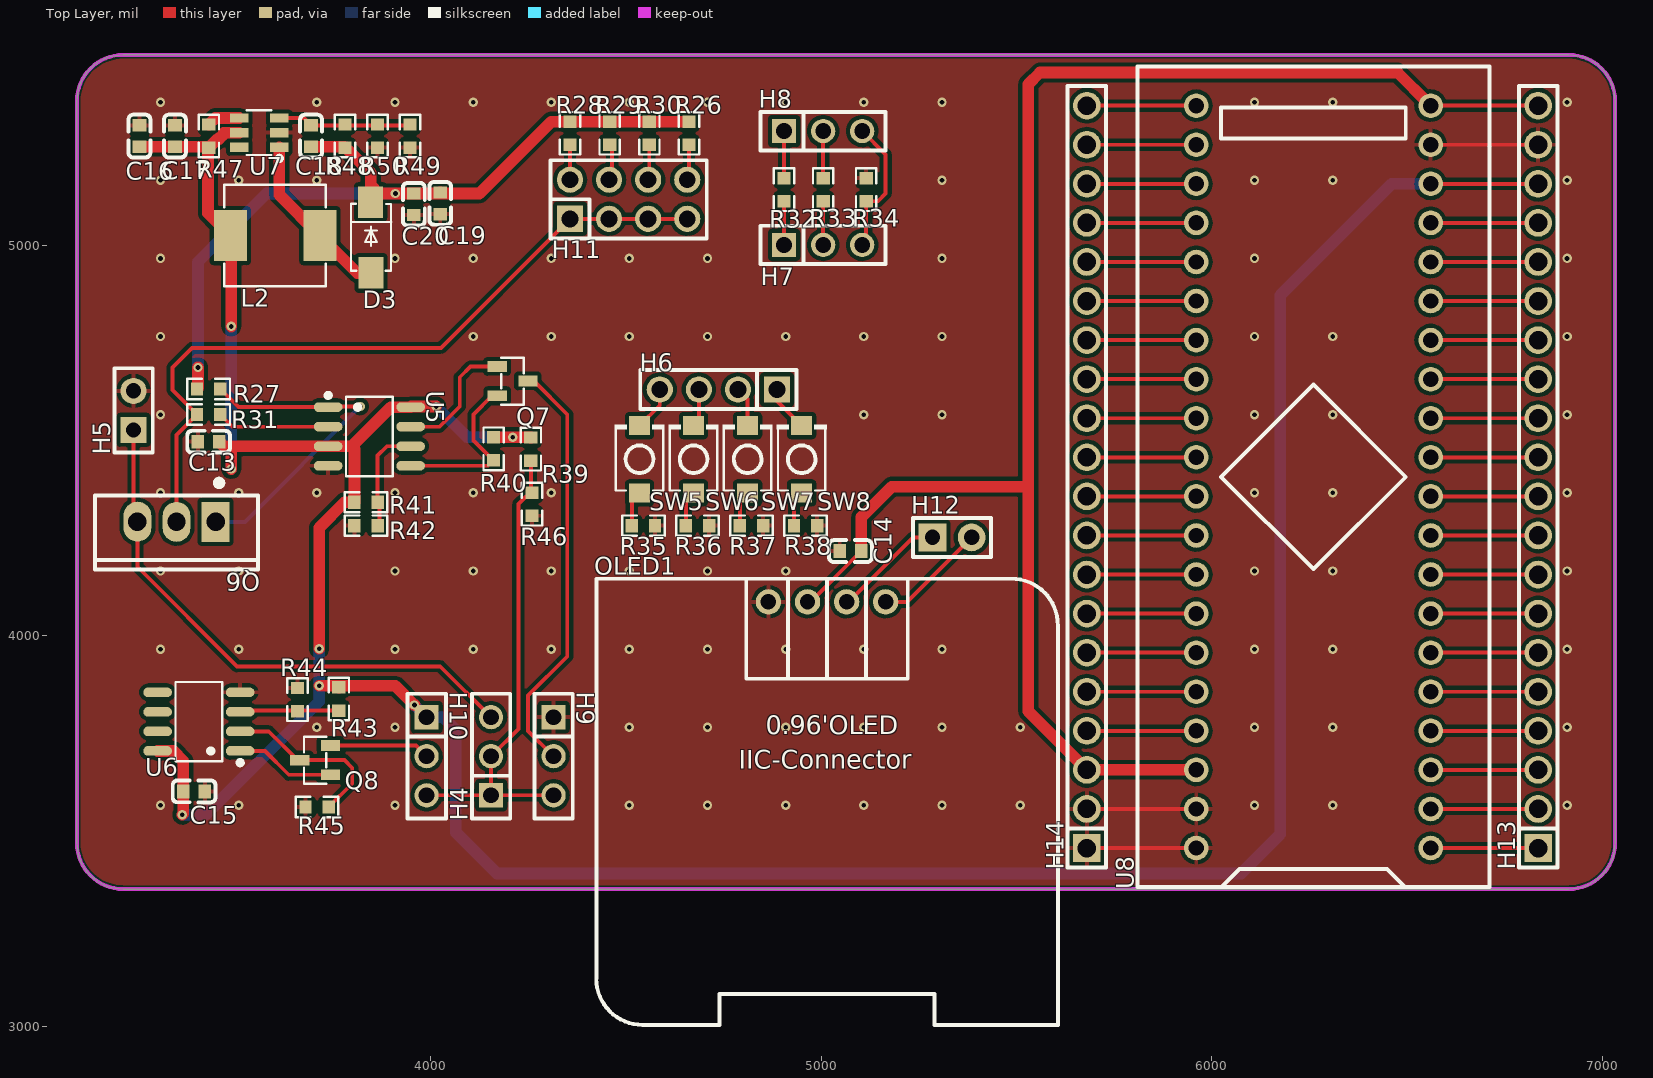
[diagram p0: Top Layer view]
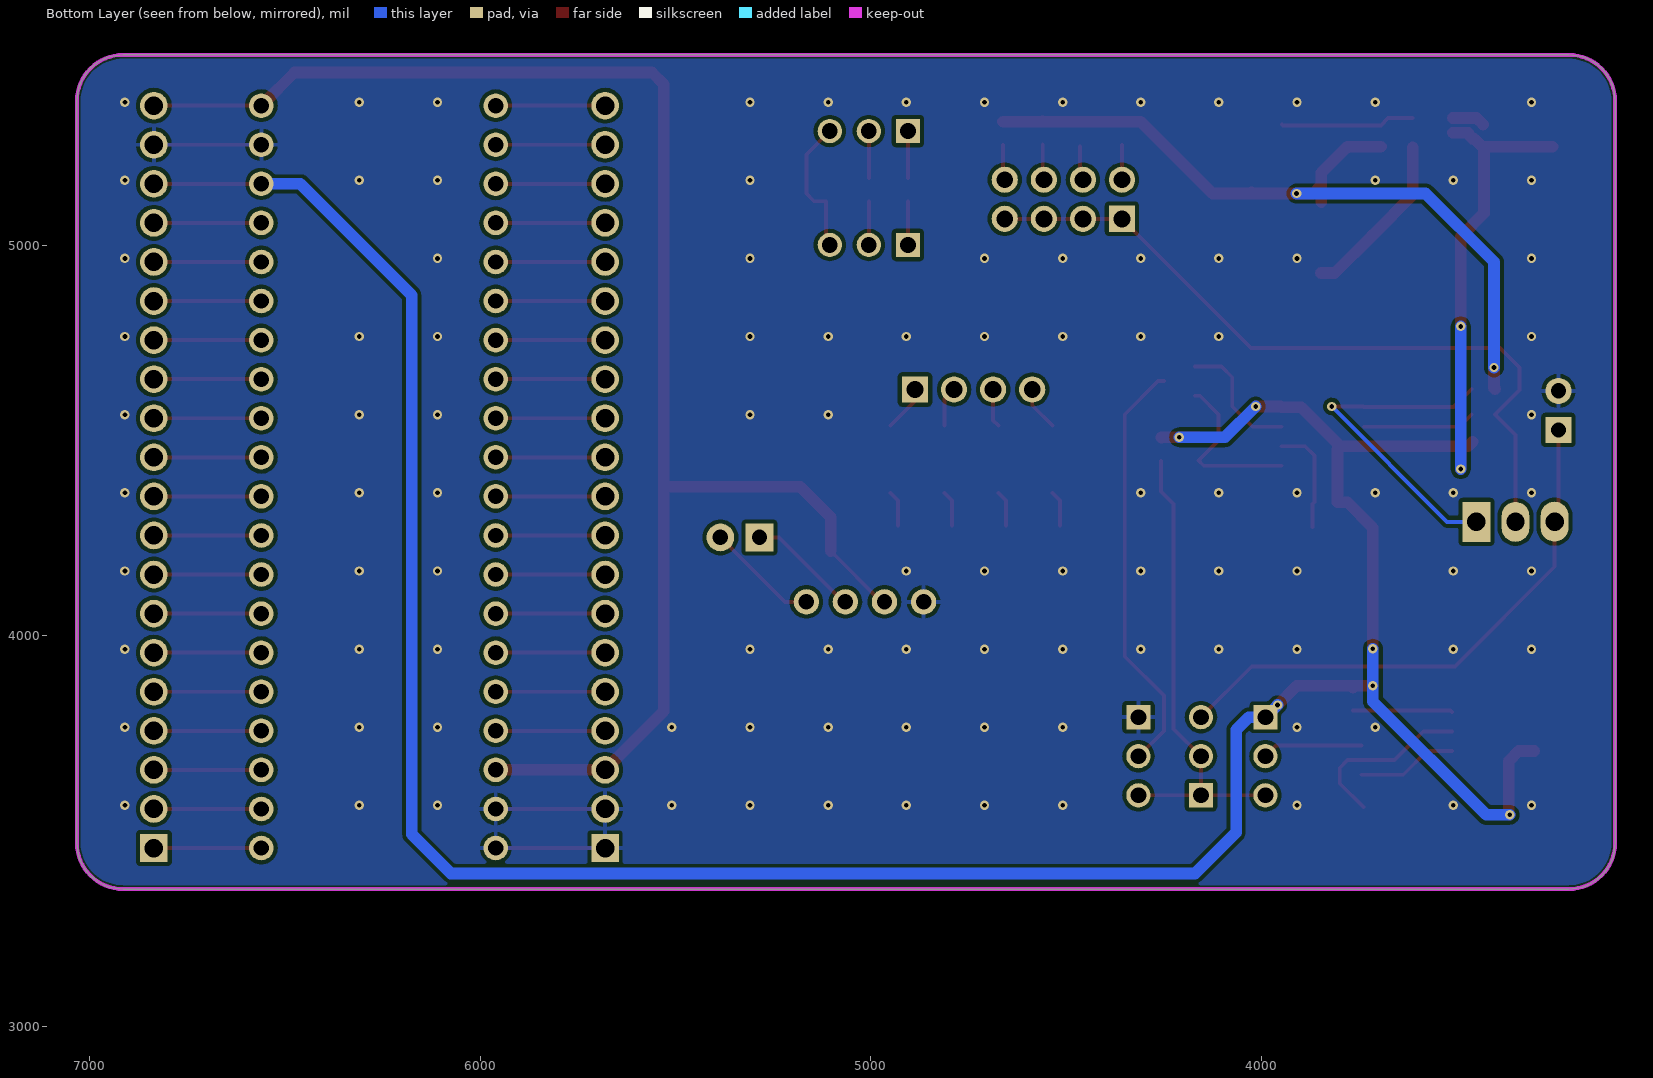
[diagram p1: Bottom Layer view, seen from below]
# Altium PCB MISC52056.pcbdoc
Units mil, origin at the board's own origin, x right, y up, seen from the top; angles counter-clockwise.
Board outline 3937.01 x 2135 mil, 2 copper layers (Top Layer, Bottom Layer), stack 62.206 mil thick; 58 components, 73 nets, 224 pads, 113 vias.

## Layer stack, top to bottom
Top Solder Mask Layer: solder mask 0.394, Dk 3.3
Top Layer: signal copper 1.379
Dielectric1: surface 59.449, FR4, Dk 4.5
Bottom Layer: signal copper 1.378
Bottom Solder Mask Layer: solder mask 0.394, Dk 3.3

## Board outline
3213.11,5486.61 ccw(c3213.11,5368.5) 3095,5368.5 3095,3469.72 ccw(c3213.11,3469.72) 3213.11,3351.61 6913.9,3351.61 ccw(c6913.9,3469.72) 7032.01,3469.72 7032.01,5368.5 ccw(c6913.9,5368.5) 6913.9,5486.61

## Design rules (kind name [scope] priority, off if disabled: settings)
BoardOutlineClearance copperThickness2oz_1 [All] p2 off: genericclearance=7.99 ignorepadtopadclearanceinfootprint=FALSE except(0: Arc-SplitContinuation Track-SplitContinuation SMDPad-SplitContinuation THPad-SplitContinuation Via-SplitContinuation Fill-SplitContinuation Region-SplitContinuation Poly-SplitContinuation Text-SplitContinuation Hole-SplitContinuation; 5.98: Arc-CutoutEdge Track-CutoutEdge SMDPad-CutoutEdge THPad-CutoutEdge Via-CutoutEdge Text-CutoutEdge; 6.9: Hole-OutlineEdge Hole-CutoutEdge; 10: Poly-OutlineEdge Poly-CutoutEdge; 11.81: Arc-OutlineEdge Track-OutlineEdge SMDPad-OutlineEdge THPad-OutlineEdge Via-OutlineEdge Fill-OutlineEdge Region-OutlineEdge Text-OutlineEdge Fill-CutoutEdge Region-CutoutEdge)
BoardOutlineClearance Plane_innerPlane_1 [All] p4 off: genericclearance=4.02 ignorepadtopadclearanceinfootprint=FALSE except(0: Arc-SplitContinuation Track-SplitContinuation SMDPad-SplitContinuation THPad-SplitContinuation Via-SplitContinuation Fill-SplitContinuation Region-SplitContinuation Poly-SplitContinuation Text-SplitContinuation Hole-SplitContinuation; 5.98: Arc-CutoutEdge Track-CutoutEdge SMDPad-CutoutEdge THPad-CutoutEdge Via-CutoutEdge Text-CutoutEdge; 6.9: Hole-OutlineEdge Hole-CutoutEdge; 10: Poly-OutlineEdge Poly-CutoutEdge; 11.81: Arc-OutlineEdge Track-OutlineEdge SMDPad-OutlineEdge THPad-OutlineEdge Via-OutlineEdge Fill-OutlineEdge Region-OutlineEdge Text-OutlineEdge Fill-CutoutEdge Region-CutoutEdge)
BoardOutlineClearance Copper_copperRegion_1 [All] p6 off: genericclearance=4.02 ignorepadtopadclearanceinfootprint=FALSE except(0: Arc-SplitContinuation Track-SplitContinuation SMDPad-SplitContinuation THPad-SplitContinuation Via-SplitContinuation Fill-SplitContinuation Region-SplitContinuation Poly-SplitContinuation Text-SplitContinuation Hole-SplitContinuation; 5.98: Arc-CutoutEdge Track-CutoutEdge SMDPad-CutoutEdge THPad-CutoutEdge Via-CutoutEdge Text-CutoutEdge; 6.9: Hole-OutlineEdge Hole-CutoutEdge; 10: Poly-OutlineEdge Poly-CutoutEdge; 11.81: Arc-OutlineEdge Track-OutlineEdge SMDPad-OutlineEdge THPad-OutlineEdge Via-OutlineEdge Fill-OutlineEdge Region-OutlineEdge Text-OutlineEdge Fill-CutoutEdge Region-CutoutEdge)
BoardOutlineClearance copperThickness1oz_1 [All] p8: genericclearance=4.02 ignorepadtopadclearanceinfootprint=FALSE except(0: Arc-SplitContinuation Track-SplitContinuation SMDPad-SplitContinuation THPad-SplitContinuation Via-SplitContinuation Fill-SplitContinuation Region-SplitContinuation Poly-SplitContinuation Text-SplitContinuation Hole-SplitContinuation; 5.98: Arc-CutoutEdge Track-CutoutEdge SMDPad-CutoutEdge THPad-CutoutEdge Via-CutoutEdge Text-CutoutEdge; 6.9: Hole-OutlineEdge Hole-CutoutEdge; 10: Poly-OutlineEdge Poly-CutoutEdge; 11.81: Arc-OutlineEdge Track-OutlineEdge SMDPad-OutlineEdge THPad-OutlineEdge Via-OutlineEdge Fill-OutlineEdge Region-OutlineEdge Text-OutlineEdge Fill-CutoutEdge Region-CutoutEdge)
Clearance copperThickness2oz [All] p1 off: gap=7.99 ignorepadtopadclearanceinfootprint=FALSE except(5.98: SMDPad-Track SMDPad-SMDPad THPad-Track SMDPad-THPad THPad-THPad Track-Via SMDPad-Via THPad-Via Via-Via Fill-SMDPad Region-SMDPad Fill-THPad Region-THPad Fill-Via Region-Via Fill-Fill Fill-Region Region-Region Arc-Track Arc-SMDPad Arc-THPad Arc-Via Fill-Arc Region-Arc Arc-Arc Text-Track SMDPad-Text Text-THPad Text-Via Fill-Text Region-Text Arc-Text Text-Text; 6.9: Hole-Track Hole-SMDPad Hole-THPad Hole-Via Fill-Hole Region-Hole Hole-Arc Hole-Text; 10: Poly-Track Poly-SMDPad Poly-THPad Poly-Via Poly-Fill Poly-Region Poly-Poly Poly-Arc Poly-Text Poly-Hole; 11.81: Fill-Track Region-Track)
Clearance Plane_innerPlane [All] p3 off: gap=4.02 ignorepadtopadclearanceinfootprint=FALSE except(5.98: SMDPad-Track SMDPad-SMDPad THPad-Track SMDPad-THPad THPad-THPad Track-Via SMDPad-Via THPad-Via Via-Via Fill-SMDPad Region-SMDPad Fill-THPad Region-THPad Fill-Via Region-Via Fill-Fill Fill-Region Region-Region Arc-Track Arc-SMDPad Arc-THPad Arc-Via Fill-Arc Region-Arc Arc-Arc Text-Track SMDPad-Text Text-THPad Text-Via Fill-Text Region-Text Arc-Text Text-Text; 6.9: Hole-Track Hole-SMDPad Hole-THPad Hole-Via Fill-Hole Region-Hole Hole-Arc Hole-Text; 10: Poly-Track Poly-SMDPad Poly-THPad Poly-Via Poly-Fill Poly-Region Poly-Poly Poly-Arc Poly-Text Poly-Hole; 11.81: Fill-Track Region-Track)
Clearance Copper_copperRegion [All] p5 off: gap=4.02 ignorepadtopadclearanceinfootprint=FALSE except(5.98: SMDPad-Track SMDPad-SMDPad THPad-Track SMDPad-THPad THPad-THPad Track-Via SMDPad-Via THPad-Via Via-Via Fill-SMDPad Region-SMDPad Fill-THPad Region-THPad Fill-Via Region-Via Fill-Fill Fill-Region Region-Region Arc-Track Arc-SMDPad Arc-THPad Arc-Via Fill-Arc Region-Arc Arc-Arc Text-Track SMDPad-Text Text-THPad Text-Via Fill-Text Region-Text Arc-Text Text-Text; 6.9: Hole-Track Hole-SMDPad Hole-THPad Hole-Via Fill-Hole Region-Hole Hole-Arc Hole-Text; 10: Poly-Track Poly-SMDPad Poly-THPad Poly-Via Poly-Fill Poly-Region Poly-Poly Poly-Arc Poly-Text Poly-Hole; 11.81: Fill-Track Region-Track)
Clearance copperThickness1oz [All] p7: gap=4.02 ignorepadtopadclearanceinfootprint=FALSE except(5.98: SMDPad-Track SMDPad-SMDPad THPad-Track SMDPad-THPad THPad-THPad Track-Via SMDPad-Via THPad-Via Via-Via Fill-SMDPad Region-SMDPad Fill-THPad Region-THPad Fill-Via Region-Via Fill-Fill Fill-Region Region-Region Arc-Track Arc-SMDPad Arc-THPad Arc-Via Fill-Arc Region-Arc Arc-Arc Text-Track SMDPad-Text Text-THPad Text-Via Fill-Text Region-Text Arc-Text Text-Text; 6.9: Hole-Track Hole-SMDPad Hole-THPad Hole-Via Fill-Hole Region-Hole Hole-Arc Hole-Text; 10: Poly-Track Poly-SMDPad Poly-THPad Poly-Via Poly-Fill Poly-Region Poly-Poly Poly-Arc Poly-Text Poly-Hole; 11.81: Fill-Track Region-Track)
DiffPairsRouting differentialPair [All] p1: maxlimit=6 minlimit=6 mostfreqgap=6 toplayer_minwidth=5 toplayer_prefwidth=10 toplayer_maxwidth=100 toplayer_mingap=6 toplayer_prefgap=6 toplayer_maxgap=6 bottomlayer_minwidth=5 bottomlayer_prefwidth=10 bottomlayer_maxwidth=100 bottomlayer_mingap=6 bottomlayer_prefgap=6 bottomlayer_maxgap=6 maxuncoupledlength=10
HoleToHoleClearance otherClearance [All] p1: gap=11.81 allowstackedmicrovias=TRUE
Length netLength [All] p1: minlimit=0 maxlimit=0
PasteMaskExpansion pasteMaskExpansion [All] p1: expansion=0
PlaneConnect innerPlane [All] p1: planeconnectstyle=Relief reliefexpansion=20 reliefentries=4 reliefconductorwidth=10 reliefairgap=10
PolygonConnect copperRegion [All] p1: connectstyle=Relief reliefconductorwidth=10 reliefentries=4 polygonreliefangle="90 Angle" airgapwidth=10 via.connectstyle=Relief via.reliefconductorwidth=10 via.reliefentries=4 via.polygonreliefangle="90 Angle" via.airgapwidth=10
RoutingVias viaSize [All] p1: holewidth=12.01 width=24.02 viastyle="Through Hole" minholewidth=11.81 minwidth=19.68 maxholewidth=248.03 maxwidth=393.7
SolderMaskExpansion solderMaskExpansion [IsVia] p1: expansion=-1000 istentingtop=TRUE
SolderMaskExpansion solderMaskExpansion [All] p2: expansion=2 istentingtop=FALSE
Width copperThickness2oz_2 [All] p1 off: maxlimit=100 minlimit=8 preferedwidth=10
Width copperThickness1oz_2 [All] p2: maxlimit=100 minlimit=5 preferedwidth=10

## Components (designator, comment, footprint, x,y, rotation, side; value= is the part's Value field where it differs from the comment)
C13 "104" C0603 3432.19,4496.61 r0 top
C14 "10uf" C0603 5075,4216.61 r180 top
C15 "100nF" C0603 3395,3601.61 r180 top
C16 "106" C0603 3255,5278.81 r90 top
C17 "104" C0603 3345.9,5278.81 r90 top
C18 "100pF" C0603 3694.41,5278.81 r90 top
C19 "10UF" C0603 4025,5106.61 r270 top
C20 "104" C0603 3957.38,5104.15 r270 top
D3 "SS36" SMA_L4.3-W2.6-LS5.0-FD 3847.38,5019.15 r90 top
H4 "" HDR-TH_3P-P2.54-V-F 4155,3691.61 r90 top
H5 "" HDR-TH_2P-P2.54-V-F 3240,4576.61 r90 top
H6 "" HDR-TH_4P-P2.54-V-M 4736.91,4630.16 r180 top
H7 "" HDR-TH_3P-P2.54-V-F 5005,5000.16 r0 top
H8 "" HDR-TH_3P-P2.54-V-F 5005,5291.61 r0 top
H9 "" HDR-TH_3P-P2.54-V-F 4315,3691.61 r270 top
H10 "" HDR-TH_3P-P2.54-V-F 3990,3691.61 r270 top
H11 "" HDR-TH_8P-P2.54-V-M-R2-C4-S2.54 4507.15,5117.06 r0 top
H12 "" HDR-TH_2P-P2.54-V-M-1 5335,4251.61 r0 top
H13 "" HDR-TH_20P-P2.54-V-M-1 6835,4406.61 r90 top
H14 "" HDR-TH_20P-P2.54-V-M-1 5680,4406.61 r90 top
L2 "22uH" IND-SMD_L7.1-W6.6 3602.38,5024.15 r0 top
OLED1 "" 0.96OLED_4P 5015,4086.61 r0 top
Q6 "2N6804" TO-220-3_L10.0-W4.5-P2.54-L 3350,4291.61 r180 top
Q7 "SS8550" SOT-23-3_L2.9-W1.3-P1.90-LS2.4-BR 4210,4651.61 r180 top
Q8 "SS8550" SOT-23-3_L2.9-W1.3-P1.90-LS2.4-BR 3704.79,3681.45 r0 top
R26 "100K" R0603 4661.56,5286.09 r90 top
R27 "1K" R0603 3432.19,4631.61 r180 top
R28 "200" R0603 4357.07,5286.09 r90 top
R29 "2K" R0603 4458.57,5286.09 r90 top
R30 "20K" R0603 4560.06,5286.09 r90 top
R31 "1K" R0603 3432.19,4566.09 r0 top
R32 "100" R0603 4905,5141.61 r270 top
R33 "100" R0603 5005,5141.61 r270 top
R34 "100" R0603 5115,5141.61 r90 top
R35 "100" R0603 4545,4281.61 r0 top
R36 "100" R0603 4683.33,4281.61 r0 top
R37 "100" R0603 4821.67,4281.61 r0 top
R38 "100" R0603 4960,4281.61 r0 top
R39 "1K" R0603 4256.99,4477.59 r90 top
R40 "250K" R0603 4161.56,4478.27 r90 top
R41 "10K" R0603 3835,4341.61 r180 top
R42 "10K" R0603 3835,4281.61 r0 top
R43 "10K" R0603 3765.59,3838.09 r90 top
R44 "10K" R0603 3659.79,3836.45 r270 top
R45 "250K" R0603 3709.79,3561.45 r0 top
R46 "1K" R0603 4260,4336.61 r270 top
R47 "1K" R0603 3432.86,5278.81 r270 top
R48 "1K" R0603 3781.36,5278.81 r90 top
R49 "9.1K" R0603 3947.38,5278.81 r90 top
R50 "75K" R0603 3864.37,5278.81 r90 top
SW5 "TS-1088-AR02016" SW-SMD_L3.9-W3.0-P4.45 4535,4451.61 r90 top
SW6 "TS-1088-AR02016" SW-SMD_L3.9-W3.0-P4.45 4673.33,4451.61 r90 top
SW7 "TS-1088-AR02016" SW-SMD_L3.9-W3.0-P4.45 4811.67,4451.61 r90 top
SW8 "TS-1088-AR02016" SW-SMD_L3.9-W3.0-P4.45 4950,4451.61 r90 top
U5 "LM358DTR(XBLW)" SOIC-8_L4.9-W4.0-P1.27-LS6.0-BL 3843.71,4509.93 r270 top
U6 "LM358DTR(XBLW)" SOIC-8_L4.9-W4.0-P1.27-LS6.0-BL 3407.32,3780.21 r90 top
U7 "MT3608L" SOT-23-6_L2.9-W1.6-P0.95-LS2.8-BL_3 3561.66,5287.52 r90 top
U8 "STM32F103C8T6-Card" CONN-TH_L53.3-W22.9_STM32F103C8T6-CARD 6260,4406.61 r90 top

## Footprints (in the part's own frame and the unit in brackets; to place one, negate y for a bottom-side part, rotate by r counter-clockwise, add the part's x,y. Pads: shape width x height; smd on the part's side, far side on the other; paste and mask are expansions set on the pad)
0.96OLED_4P [mm]
  round 1.65 hole 1 copper offset 0,0: 1(-3.81,-0.001) 2(-1.27,0.002) 3(1.27,0.002) 4(3.81,0.002)
  silkscreen extent -15,-27.5 15,1.5
C0603 [mm]
  rect 0.8x0.9 smd: 1(-0.7,0) 2(0.7,0)
  silkscreen extent -1.39,-0.71 1.39,0.71
CONN-TH_L53.3-W22.9_STM32F103C8T6-CARD [mm]
  round 1.6 hole 1: 1(-24.13,-7.62) 2(-21.59,-7.62) 3(-19.05,-7.62) 4(-16.51,-7.62) 5(-13.97,-7.62) 6(-11.43,-7.62) 7(-8.89,-7.62) 8(-6.35,-7.62) 9(-3.81,-7.62) 10(-1.27,-7.62) 11(1.27,-7.62) 12(3.81,-7.62) 13(6.35,-7.62) 14(8.89,-7.62) 15(11.43,-7.62) 16(13.97,-7.62) 17(16.51,-7.62) 18(19.05,-7.62) 19(21.59,-7.62) 20(24.13,-7.62) 21(24.13,7.62) 22(21.59,7.62) 23(19.05,7.62) 24(16.51,7.62) 25(13.97,7.62) 26(11.43,7.62) 27(8.89,7.62) 28(6.35,7.62) 29(3.81,7.62) 30(1.27,7.62) 31(-1.27,7.62) 32(-3.81,7.62) 33(-6.35,7.62) 34(-8.89,7.62) 35(-11.43,7.62) 36(-13.97,7.62) 37(-16.51,7.62) 38(-19.05,7.62) 39(-21.59,7.62) 40(-24.13,7.62)
  silkscreen extent -26.67,-11.43 26.67,11.43
HDR-TH_2P-P2.54-V-F [mm]
  rect 1.7x1.7 hole 1: 1(-1.27,0)
  round 1.7 hole 1: 2(1.27,0)
  silkscreen extent -2.74,-1.25 2.74,1.25
HDR-TH_2P-P2.54-V-M-1 [mm]
  rect 1.8x1.8 hole 1: 1(-1.27,0)
  round 1.8 hole 1: 2(1.27,0)
  silkscreen extent -2.54,-1.27 2.54,1.27
HDR-TH_3P-P2.54-V-F [mil]
  rect 62x62 hole 40.16: 1(-100,0)
  round 62 hole 40.16: 2(0,0) 3(100,0)
  silkscreen extent -160,-49 160,49
HDR-TH_4P-P2.54-V-M [mm]
  rect 1.7x1.7 hole 1.1: 1(-3.81,0)
  round 1.7 hole 1.1: 2(-1.27,0) 3(1.27,0) 4(3.81,0)
  silkscreen extent -5.08,-1.27 5.08,1.27
HDR-TH_8P-P2.54-V-M-R2-C4-S2.54 [mm]
  rect 1.7x1.7 hole 1.1: 1(-3.81,-1.27)
  round 1.7 hole 1.1: 2(-3.81,1.27) 3(-1.27,-1.27) 4(-1.27,1.27) 5(1.27,-1.27) 6(1.27,1.27) 7(3.81,-1.27) 8(3.81,1.27)
  silkscreen extent -5.08,-2.54 5.08,2.54
HDR-TH_20P-P2.54-V-M-1 [mm]
  rect 1.8x1.8 hole 1.2: 1(-24.13,0)
  round 1.8 hole 1.2: 2(-21.59,0) 3(-19.05,0) 4(-16.51,0) 5(-13.97,0) 6(-11.43,0) 7(-8.89,0) 8(-6.35,0) 9(-3.81,0) 10(-1.27,0) 11(1.27,0) 12(3.81,0) 13(6.35,0) 14(8.89,0) 15(11.43,0) 16(13.97,0) 17(16.51,0) 18(19.05,0) 19(21.59,0) 20(24.13,0)
  silkscreen extent -25.4,-1.25 25.4,1.25
IND-SMD_L7.1-W6.6 [mm]
  rect 2.15x3.32 smd: 1(-2.913,0) 2(2.913,0)
  silkscreen extent -3.3,-3.3 3.3,3.3
R0603 [mil]
  rect 31.75x34.02 smd paste-3937.01 mask+2: 1(-29.66,0) 2(29.66,0)
  silkscreen extent -55,-26 55,26
SMA_L4.3-W2.6-LS5.0-FD [mm]
  rect 2.046x1.62 smd: 1(-2.304,-0.009) 2(2.304,0.009)
  silkscreen extent -2.17,-1.32 2.19,1.29
SOIC-8_L4.9-W4.0-P1.27-LS6.0-BL [mm]
  oval 0.63x1.865 smd: 1(-1.905,-2.682) 2(-0.635,-2.682) 3(0.635,-2.682) 4(1.905,-2.682) 5(1.905,2.682) 6(0.635,2.682) 7(-0.635,2.682) 8(-1.905,2.682)
  silkscreen extent -2.82,-2.83 2.58,1.52
SOT-23-3_L2.9-W1.3-P1.90-LS2.4-BR [mm]
  rect 1.25x0.7 smd: 1(1,-0.95) 2(1,0.95) 3(-1,0)
  silkscreen extent -0.73,-1.53 0.73,1.53
SOT-23-6_L2.9-W1.6-P0.95-LS2.8-BL_3 [mm]
  rect 0.6x1.2 smd: 1(-0.95,-1.3) 2(0,-1.3) 3(0.95,-1.3) 4(0.95,1.3) 5(0,1.3) 6(-0.95,1.3)
  silkscreen extent -1.82,-1.45 1.45,0.8
SW-SMD_L3.9-W3.0-P4.45 [mm]
  rect 1.23x1.36 smd: 1(-2.185,0) 2(2.185,0)
  silkscreen extent -2.03,-1.62 2.25,1.62
TO-220-3_L10.0-W4.5-P2.54-L [mm]
  rect 1.8x2.6 hole 1.2: 1(-2.54,0.005)
  oval 1.8x2.6 hole 1.2: 2(0,0.005)
  oval 1.8x2.6 hole 1.2 copper offset 0,0: 3(2.54,-0.005)
  silkscreen extent -5.3,-2.73 5.3,3.09

## Via types
v1: diameter 24.02, hole 12, Top Layer to Bottom Layer, 113 vias

## Nets (pads, with @x,y where several pads share a name; then routed paths per layer and width w, separated by ;. In a path a pad name is that pad's centre, name@x,y a point inside that pad or via, vN(x,y) a via of type N, cw(c..) or ccw(c..) an arc to the next point about the centre after c; other vN are vias at no path point)
3V3: C14.1 H13.20 H14.3 OLED1.2 U8.20 U8.38 | length 4185.8
  Top Layer w10: OLED1.2 4972.61,4086.66 C14.1 ; U8.20 H13.20
  Top Layer w30: C14.1 5102.56,4303.71 5180.37,4381.52 5530,4381.52 ; U8.38 H14.3 5530,3806.61 5530,4381.52 ; U8.20@6555,5356.61 6555,5361.61 6475,5441.61 5560,5441.61 5530,5411.61 5530,4381.52
8V: C18.1 C19.1 C20.1 D3.2 R26.2 R27.2 R28.2 R29.2 R30.2 R48.1 | length 2065.5
  Top Layer w30: R27.2 3405,4634.08 v1(3405,4686.61) ; C18.1 R48.1@3779.27,5251.25 ; R48.1 R48.1@3779.27,5251.25 ; D3.2 3847.01,5152.73 ; C19.1 C19.1@4022.54,5131.71 ; R30.2@4560,5316.27 R30.2@4559.48,5315.75 ; R26.2 R30.2 R30.2@4559.48,5315.75 ; R48.1@3779.27,5251.25 3780.36,5251.25 3847.01,5184.6 3847.01,5152.73 ; 3847.01,5152.73 3868.03,5131.71 v1(3910.32,5131.71) C20.1 C19.1@4022.54,5131.71 ; C19.1@4022.54,5131.71 4125.1,5131.71 4309.14,5315.75 R28.2 R29.2 R30.2@4559.48,5315.75
  Bottom Layer w30: v1(3405,4686.61) 3405,4956.61 3580.1,5131.71 v1(3910.32,5131.71)
$1N10: R31.2 U5.2 | length 289.2
  Top Layer w10: R31.2 3493.01,4534.93 U5.2
$1N11: H11.1 H11.3 H11.5 H11.7 Q6.2 R31.1 | length 1917.6
  Top Layer w10: Q6.2 3350.01,4513.56 R31.1 3340,4628.62 3340,4686.61 3390,4736.61 4026.71,4736.61 H11.1 H11.3 H11.5 H11.7
$1N17: Q6.1 R27.1 U5.1 | length 870.5
  Top Layer w10: R27.1 3508.54,4584.93 U5.1 3739.78,4586.61 v1(3820,4586.61)
  Bottom Layer w10: Q6.1 3524.8,4291.42 v1(3820,4586.61)
$1N18: H11.2 R28.1 | length 89.4
  Top Layer w10: R28.1 4357.15,5256.35 H11.2
$1N19: H11.4 R29.1 | length 88.1
  Top Layer w10: H11.4 4465,5174.91 R29.1@4465,5251.95
$1N20: H11.8 R26.1 | length 91.2
  Top Layer w10: H11.8 4661.56,5171.47 R26.1
$1N21: H11.6 R30.1 | length 91.1
  Top Layer w10: H11.6 4560,5169.91 R30.1@4560,5256.95
$1N29: Q7.1 U5.7 | length 329.1
  Top Layer w10: U5.7 4023.32,4534.93 4075,4586.61 4075,4661.61 4102.4,4689.01 Q7.1
$1N30: R41.1 R42.2 U5.6 | length 279.8
  Top Layer w10: R42.2@3869.38,4277.85 3869.38,4336.89 R41.1 3864.66,4461.27 3888.32,4484.93 U5.6
$1N31: H9.2 Q7.3 | length 1079.2
  Top Layer w10: Q7.3 4265,4651.61 4350,4566.61 4350,3946.61 4250,3846.61 4250,3756.61 H9.2
$1N42: Q8.3 R45.2 U6.2 | length 450.7
  Top Layer w10: U6.2 3586.03,3755.21 3659.79,3681.45 Q8.3 3779.79,3681.45 3799.79,3661.45 3799.79,3621.79 R45.2
$1N44: R43.1 R44.2 U6.3 | length 254
  Top Layer w10: U6.3 3516.15,3808.43 R43.1
$1N46: Q8.1 U6.1 | length 256.6
  Top Layer w10: U6.1 3576.03,3705.21 3637.19,3644.05 Q8.1
$1N48: H10.2 Q8.2 | length 257.1
  Top Layer w10: Q8.2 3962.77,3718.85 H10.2
$1N74: Q7.2 R40.1 U5.5 | length 437.6
  Top Layer w10: U5.5 4147.88,4434.93 R40.1 4110,4500.17 4110,4566.61 4157.6,4614.21 Q7.2
$1N77: C18.2 R48.2 R49.2 R50.2 U7.3 | length 343.1
  Top Layer w10: U7.3 3675.86,5324.92 C18.2 3945.28,5306.37 R49.2
$1N84: D3.1 L2.2 U7.1 | length 439.5
  Top Layer w30: U7.1 3612.84,5128.37 L2.2 3812.76,4928.45 D3.1
$1N85: R47.1 U7.4 | length 84.4
  Top Layer w30: R47.1 3449.3,5324.92 U7.4
$1N132: H6.4 SW5.2 | length 114
  Top Layer w10: SW5.2 4586.91,4589.54 H6.4
$1N133: H6.3 SW6.2 | length 98.1
  Top Layer w10: SW6.2 4686.91,4551.2 H6.3
$1N134: H6.2 SW7.2 | length 102.8
  Top Layer w10: H6.2 4811.67,4605.4 SW7.2
$1N135: H6.1 SW8.2 | length 118.7
  Top Layer w10: H6.1 4886.91,4600.73 SW8.2
$1N5188: H8.1 R32.1 | length 120.3
  Top Layer w10: R32.1 H8.1
$1N5193: H7.1 R32.2 | length 111.8
  Top Layer w10: H7.1 R32.2
$1N5205: H7.2 R33.2 | length 111.8
  Top Layer w10: H7.2 R33.2
$1N5211: H8.2 R33.1 | length 120.3
  Top Layer w10: R33.1 H8.2
$1N5227: H7.3 H8.3 R34.1 | length 358.9
  Top Layer w10: H7.3 5115,5010.16 R34.1 5145.34,5111.95 5165,5131.61 5165,5231.61 H8.3
$1N13950: R35.1 SW5.1 | length 92.1
  Top Layer w10: R35.1 4515.34,4345.93 SW5.1
$1N13997: R36.1 SW6.1 | length 92.1
  Top Layer w10: R36.1 4653.67,4345.93 SW6.1
$1N14044: R37.1 SW7.1 | length 92.1
  Top Layer w10: R37.1 4792.01,4345.93 SW7.1
$1N14091: R38.1 SW8.1 | length 92.1
  Top Layer w10: R38.1 4930.34,4345.93 SW8.1
$1N25561: H13.1 U8.1 | length 275
  Top Layer w10: U8.1 H13.1
$1N25563: H13.2 U8.2 | length 275
  Top Layer w10: U8.2 H13.2
$1N25565: H13.3 U8.3 | length 275
  Top Layer w10: U8.3 H13.3
$1N25567: H13.4 U8.4 | length 275
  Top Layer w10: U8.4 H13.4
$1N25569: H13.5 U8.5 | length 275
  Top Layer w10: U8.5 H13.5
$1N25571: H13.6 U8.6 | length 275
  Top Layer w10: U8.6 H13.6
$1N25573: H13.7 U8.7 | length 275
  Top Layer w10: U8.7 H13.7
$1N25575: H13.8 U8.8 | length 275
  Top Layer w10: U8.8 H13.8
$1N25577: H13.9 U8.9 | length 275
  Top Layer w10: U8.9 H13.9
$1N25579: H13.10 U8.10 | length 275
  Top Layer w10: U8.10 H13.10
$1N25581: H13.11 U8.11 | length 275
  Top Layer w10: U8.11 H13.11
$1N25583: H13.12 U8.12 | length 275
  Top Layer w10: U8.12 H13.12
$1N25585: H13.13 U8.13 | length 275
  Top Layer w10: U8.13 H13.13
$1N25587: H13.14 U8.14 | length 275
  Top Layer w10: U8.14 H13.14
$1N25589: H13.15 U8.15 | length 275
  Top Layer w10: U8.15 H13.15
$1N25591: H13.16 U8.16 | length 275
  Top Layer w10: U8.16 H13.16
$1N25593: H13.17 U8.17 | length 275
  Top Layer w10: U8.17 H13.17
$1N25755: H14.20 U8.21 | length 290
  Top Layer w10: H14.20@5670,5356.61 U8.21
$1N25757: H14.19 U8.22 | length 290
  Top Layer w10: H14.19@5670,5256.61 U8.22
$1N25759: H14.18 U8.23 | length 290
  Top Layer w10: H14.18@5670,5156.61 U8.23
$1N25761: H14.17 U8.24 | length 290
  Top Layer w10: H14.17@5670,5056.61 U8.24
$1N25763: H14.16 U8.25 | length 290
  Top Layer w10: H14.16@5670,4956.61 U8.25
$1N25765: H14.15 U8.26 | length 290
  Top Layer w10: H14.15@5670,4856.61 U8.26
$1N25767: H14.14 U8.27 | length 290
  Top Layer w10: H14.14@5670,4756.61 U8.27
$1N25769: H14.13 U8.28 | length 290
  Top Layer w10: H14.13@5670,4656.61 U8.28
$1N25771: H14.12 U8.29 | length 290
  Top Layer w10: H14.12@5670,4556.61 U8.29
$1N25773: H14.11 U8.30 | length 290
  Top Layer w10: H14.11@5670,4456.61 U8.30
$1N25775: H14.10 U8.31 | length 290
  Top Layer w10: H14.10@5670,4356.61 U8.31
$1N25777: H14.9 U8.32 | length 290
  Top Layer w10: H14.9@5670,4256.61 U8.32
$1N25779: H14.8 U8.33 | length 290
  Top Layer w10: H14.8@5670,4156.61 U8.33
$1N25781: H14.7 U8.34 | length 290
  Top Layer w10: H14.7@5670,4056.61 U8.34
$1N25783: H14.6 U8.35 | length 290
  Top Layer w10: H14.6@5670,3956.61 U8.35
$1N25785: H14.5 U8.36 | length 290
  Top Layer w10: H14.5@5670,3856.61 U8.36
$1N25787: H14.4 U8.37 | length 290
  Top Layer w10: H14.4@5670,3756.61 U8.37
+5V: C13.2 C15.2 C16.1 C17.1 H10.1 H13.18 L2.1 R39.2 R40.2 R41.2 R43.2 R47.2 U5.3 U5.8 U6.8 U7.5 U8.18 | length 8519.9
  Top Layer w10: U8.18 H13.18
  Top Layer w30: C16.1 C17.1 R47.2@3430.76,5251.25 ; U6.8 3341.4,3705.21 3367.44,3679.17 C15.2 3367.44,3544.05 v1(3365,3541.61) ; C13.2 3471.44,4484.93 3487.74,4484.93 ; v1(3490,4426.61) 3490,4482.67 3487.74,4484.93 ; v1(3490,4791.61) 3490,5021.85 L2.1 3430.76,5081.09 R47.2@3430.76,5251.25 ; U7.5 3471.22,5287.52 3470.85,5287.15 3470.85,5283.91 3458.56,5271.61 3455.32,5271.61 R47.2 R47.2@3430.76,5251.25 ; v1(3715,3871.61) R43.2@3761.73,3871.61 ; v1(3715,3966.61) 3715,4276.61 3780,4341.61 R41.2 3805.34,4477.9 3798.32,4484.93 ; R43.2 R43.2@3761.73,3871.61 ; v1(3958.95,3822.66) 3910,3871.61 R43.2@3761.73,3871.61 ; v1(4015,4586.61) 3951,4586.61 U5.8 3898.32,4584.93 3798.32,4484.93 ; R40.2 v1(4210.69,4507.93) 4256.31,4507.93 R39.2 ; 3487.74,4484.93 U5.3 3798.32,4484.93
  Bottom Layer w30: v1(3365,3541.61) 3425,3541.61 3715,3831.61 v1(3715,3871.61) v1(3715,3966.61) ; v1(3490,4426.61) v1(3490,4791.61) ; v1(3958.95,3822.66) H10.1 4032.43,3791.61 4065,3759.04 4065,3496.61 4170,3391.61 6075,3391.61 6175,3491.61 6175,4871.61 6460,5156.61 U8.18 ; v1(4015,4586.61) 4093.69,4507.93 v1(4210.69,4507.93)
GND: C13.1 C14.2 C15.1 C16.2 C17.2 C19.2 C20.2 H5.2 H9.1 H13.19 H14.1 H14.2 OLED1.1 R34.2 R35.2 R36.2 R37.2 R38.2 R42.1 R44.1 R45.1 R46.2 R49.1 R50.1 U5.4 U6.4 U7.2 U8.19 U8.39 U8.40 | length 855
  Top Layer w10: H14.1@5670,3456.61 U8.40 ; H14.2@5670,3556.61 U8.39 ; U8.19 H13.19
  other v1: 3309.1,3565.71 3509.1,3565.71 3909.1,3565.71 4509.1,3565.71 4709.1,3565.71 4909.1,3565.71 5109.1,3565.71 5309.1,3565.71 5509.1,3565.71 6109.1,3565.71 6309.1,3565.71 6909.1,3565.71 3709.1,3765.71 3909.1,3765.71 4509.1,3765.71 4709.1,3765.71 4909.1,3765.71 5109.1,3765.71 5309.1,3765.71 5509.1,3765.71 6109.1,3765.71 6309.1,3765.71 6909.1,3765.71 3309.1,3965.71 3509.1,3965.71 3909.1,3965.71 4109.1,3965.71 4309.1,3965.71 4509.1,3965.71 4709.1,3965.71 4909.1,3965.71 5109.1,3965.71 5309.1,3965.71 6109.1,3965.71 6309.1,3965.71 6909.1,3965.71 3309.1,4165.71 3509.1,4165.71 3909.1,4165.71 4109.1,4165.71 4309.1,4165.71 4509.1,4165.71 4709.1,4165.71 4909.1,4165.71 6109.1,4165.71 6309.1,4165.71 6909.1,4165.71 3309.1,4365.71 3509.1,4365.71 3709.1,4365.71 3909.1,4365.71 4109.1,4365.71 4309.1,4365.71 6109.1,4365.71 6309.1,4365.71 6909.1,4365.71 3309.1,4565.71 5109.1,4565.71 5309.1,4565.71 6109.1,4565.71 6309.1,4565.71 6909.1,4565.71 3309.1,4765.71 4109.1,4765.71 4309.1,4765.71 4509.1,4765.71 4709.1,4765.71 4909.1,4765.71 5109.1,4765.71 5309.1,4765.71 6109.1,4765.71 6309.1,4765.71 6909.1,4765.71 3309.1,4965.71 3909.1,4965.71 4109.1,4965.71 4309.1,4965.71 4509.1,4965.71 4709.1,4965.71 5309.1,4965.71 6109.1,4965.71 6909.1,4965.71 3309.1,5165.71 3509.1,5165.71 3709.1,5165.71 5309.1,5165.71 6109.1,5165.71 6309.1,5165.71 6909.1,5165.71 3309.1,5365.71 3709.1,5365.71 3909.1,5365.71 4109.1,5365.71 4309.1,5365.71 4509.1,5365.71 4709.1,5365.71 4909.1,5365.71 5109.1,5365.71 5309.1,5365.71 6109.1,5365.71 6309.1,5365.71 6909.1,5365.71
IN1: H4.3 H5.1 Q6.3 | length 1418.6
  Top Layer w10: H5.1 3240,4301.8 Q6.3 3249.99,4176.62 3505,3921.61 4025,3921.61 H4.3
NPN_C: H4.1 H4.2 H9.3 H10.3 R39.1 R46.1 | length 1223.6
  Top Layer w10: H10.3 H4.1 ; R39.1 4256.99,4368.73 4225,4336.74 4225,3761.61 H4.2 H4.1 ; H9.3 H4.1
OLED_SCL: H12.1 OLED1.3 | length 288.3
  Top Layer w10: OLED1.3 5070.05,4086.66 5235,4251.61 H12.1
OLED_SDA: H12.2 OLED1.4 | length 288.3
  Top Layer w10: OLED1.4 5220.05,4086.66 H12.2
pads on no net: U6.5 U6.6 U6.7 U7.6

## Polygon pours and split planes (outlines as drawn)
GND on Top Layer (solid, remove dead copper, pour order 0): 3000,5596.61 3000,3261.61 7181.87,3261.61 7181.87,5596.61
GND on Bottom Layer (solid, remove dead copper, pour order 2): 3010,5601.61 3010,3251.61 7170,3251.61 7170,5601.61

## Keep-outs
Board Outline Layer:
  the board outline again, w10